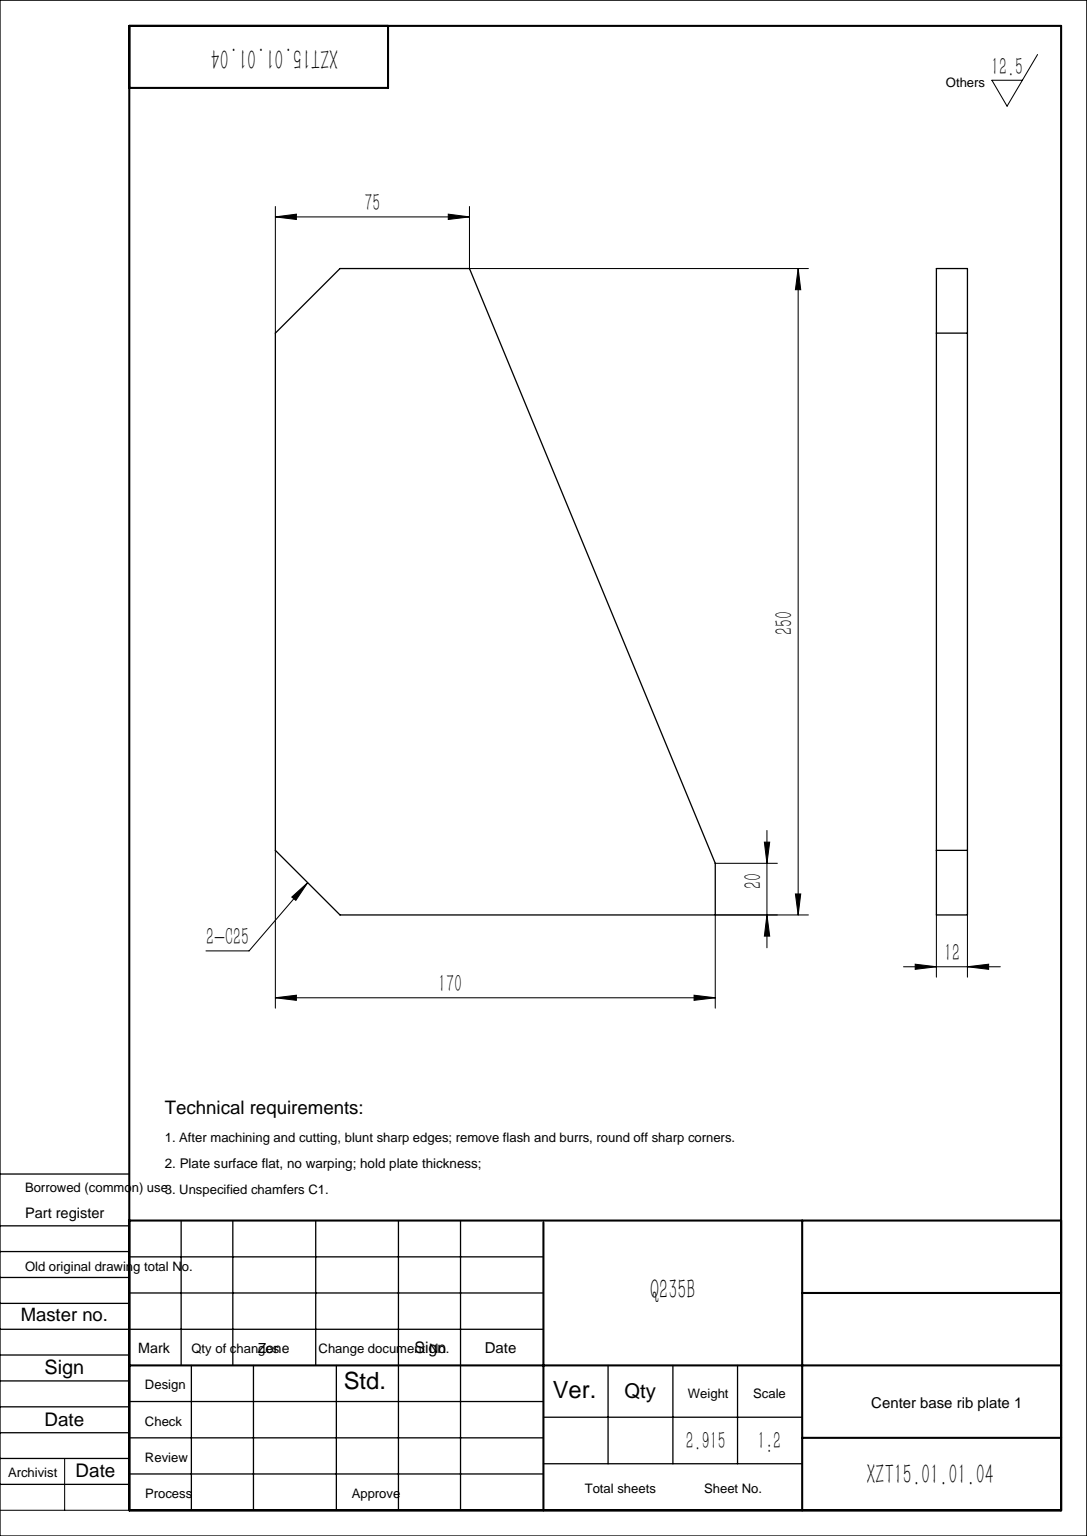
SolidWorks part; units mm, degrees
material "Q235B"
ref_plane "Front Plane" through (0, 0, 0) normal (0, 0, 1) x (1, 0, 0)
ref_plane "Top Plane" through (0, 0, 0) normal (0, 1, 0) x (1, 0, 0)
ref_plane "Right Plane" through (0, 0, 0) normal (1, 0, 0) x (0, 0, -1)
sketch "Sketch1" plane through (0, 0, 0) normal (0, 0, 1) x (1, 0, 0)
  line L0 (0, 0) -> (170, 0)
  line L1 (170, 0) -> (170, 20)
  line L2 (170, 20) -> (75, 250)
  line L3 (75, 250) -> (0, 250)
  line L4 (0, 250) -> (0, 0)
  dimension "D1" = 170
  dimension "D2" = 20
  dimension "D3" = 75
  dimension "D4" = 250
extrude "Boss-Extrude1" add sketch "Sketch1" along normal mid plane 12
chamfer "Chamfer1" distance 25 angle 45 2 edges at (0, 0, 0) (0, 250, 0)
